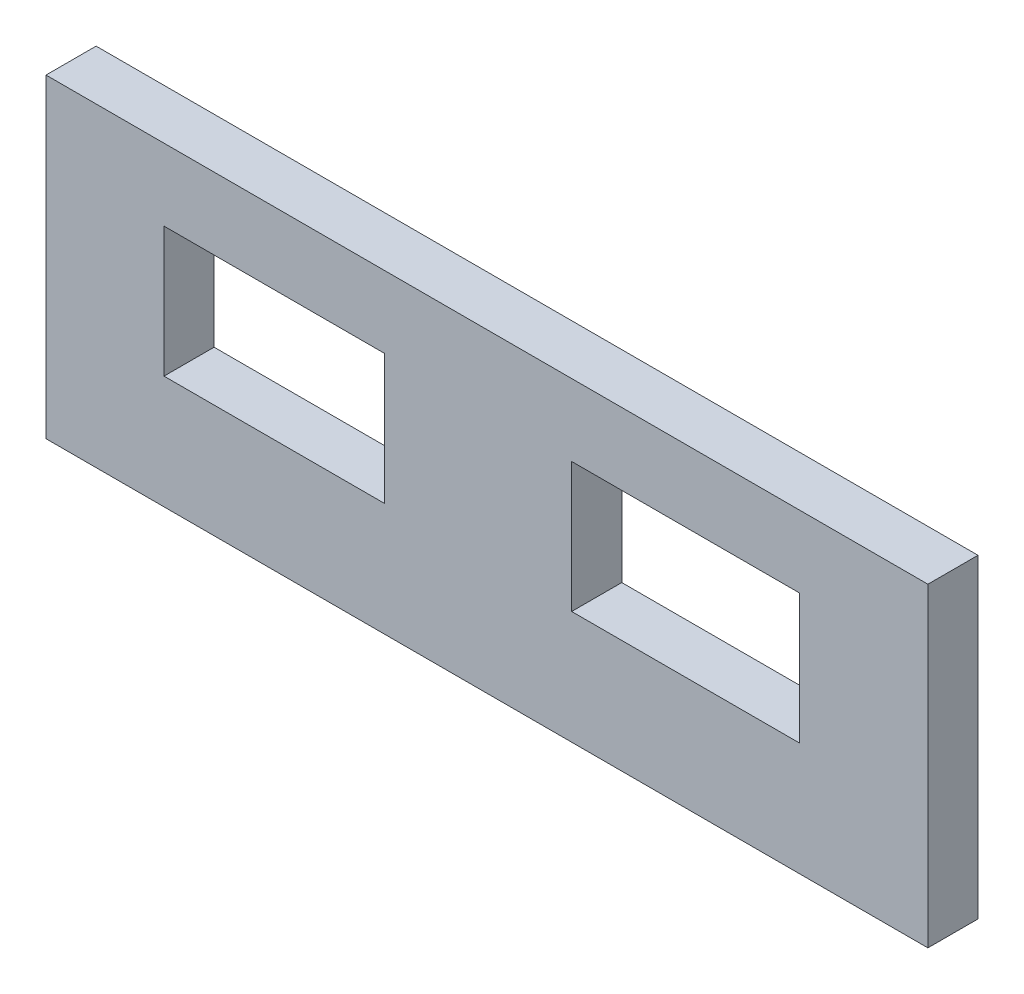
SolidWorks part; units mm, degrees
ref_plane "Front Plane" through (0, 0, 0) normal (0, 0, 1) x (1, 0, 0)
ref_plane "Top Plane" through (0, 0, 0) normal (0, 1, 0) x (1, 0, 0)
ref_plane "Right Plane" through (0, 0, 0) normal (1, 0, 0) x (0, 0, -1)
sketch "Sketch1" plane through (0, 0, 0) normal (0, 1, 0) x (1, 0, 0)
  line L1 (-308, -17.5) -> (308, -17.5)
  line L2 (-308, -17.5) -> (-308, 17.5)
  line L3 (-308, 17.5) -> (308, 17.5)
  line L4 (308, -17.5) -> (308, 17.5)
  line L5 (-308, -17.5) -> (308, 17.5) construction
  line L6 (-308, 17.5) -> (308, -17.5) construction
  point P0 (0, 0)
  point P6 (-143.3321, 17.5)
  dimension "D1" = 616
  dimension "D2" = 35
extrude "Boss-Extrude1" add sketch "Sketch1" along normal blind 220
sketch "Sketch2" plane through (0, 0, 17.5) normal (0, 0, 1) x (1, 0, 0)
  line L1 (-225.5752, 169.8419) -> (-71.6324, 169.8419)
  line L2 (-225.5752, 169.8419) -> (-225.5752, 79.078)
  line L3 (-225.5752, 79.078) -> (-71.6324, 79.078)
  line L4 (-71.6324, 169.8419) -> (-71.6324, 79.078)
  line L5 (-225.5752, 169.8419) -> (-71.6324, 79.078) construction
  line L6 (-225.5752, 79.078) -> (-71.6324, 169.8419) construction
  line L7 (59.1746, 79.078) -> (218.4565, 79.078)
  line L8 (59.1746, 79.078) -> (59.1746, 169.8419)
  line L9 (59.1746, 169.8419) -> (218.4565, 169.8419)
  line L10 (218.4565, 79.078) -> (218.4565, 169.8419)
  line L11 (59.1746, 79.078) -> (218.4565, 169.8419) construction
  line L12 (59.1746, 169.8419) -> (218.4565, 79.078) construction
  point P0 (-148.6038, 124.46)
  point P5 (138.8155, 124.46)
extrude "Cut-Extrude1" cut sketch "Sketch2" against normal through all
